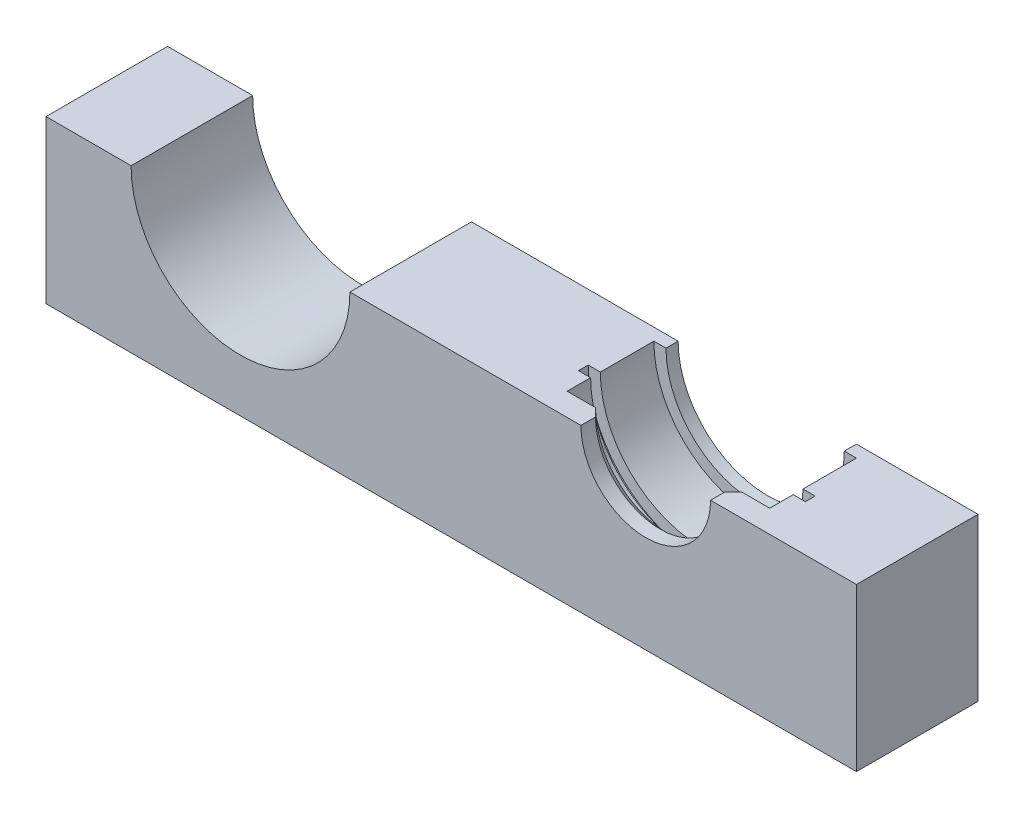
from build123d import *

# Parameters (mm, degrees)
SKETCH1_W               = 1000
SKETCH1_H               = 200
BOSS_EXTRUDE1_DEPTH     = 150
CUT_EXTRUDE1_DEPTH      = 1031.776406404
CUT_EXTRUDE1_DEPTH_BACK = 1031.776406404
SKETCH2_R               = 135
SKETCH2_R_2             = 80
CHAMFER1_SIZE           = 10


with BuildPart() as part:
    # Sketch1 → Boss-Extrude1 (new body)
    with BuildSketch(Plane.XY):
        with Locations((500, -100)):
            Rectangle(SKETCH1_W, SKETCH1_H)
    extrude(amount=BOSS_EXTRUDE1_DEPTH)

    # Sketch2 → Cut-Extrude1 (cut, two sides: drawn at the far end of the back side and taken through both)
    with BuildSketch(Plane.XY.offset(150).offset(-CUT_EXTRUDE1_DEPTH_BACK)):
        with Locations((240, 0)):
            Circle(SKETCH2_R)
        with Locations((740, 0)):
            Circle(SKETCH2_R_2)
    extrude(amount=CUT_EXTRUDE1_DEPTH + CUT_EXTRUDE1_DEPTH_BACK, mode=Mode.SUBTRACT)

    # Sketch3 → Cut-Revolve1 (revolve, cut)
    with BuildSketch(Plane(origin=(0, 0, 0), x_dir=(1, 0, 0), z_dir=(0, 1, 0))):
        Polygon((740, -150), (660, -150), (660, -122), (615, -122), (615, -93), (600, -93), (600, -81), (615, -81), (615, -15), (630, -15), (630, 0), (740, 0), align=None)
    revolve(axis=Axis((740, 0, 0), (0, 0, 1)), mode=Mode.SUBTRACT)

    # Chamfer1
    chamfer1_edges = [part.edges().sort_by_distance(p)[0] for p in [
        (740, -80, 122),
    ]]
    chamfer(chamfer1_edges, length=CHAMFER1_SIZE)


solid = part.part
